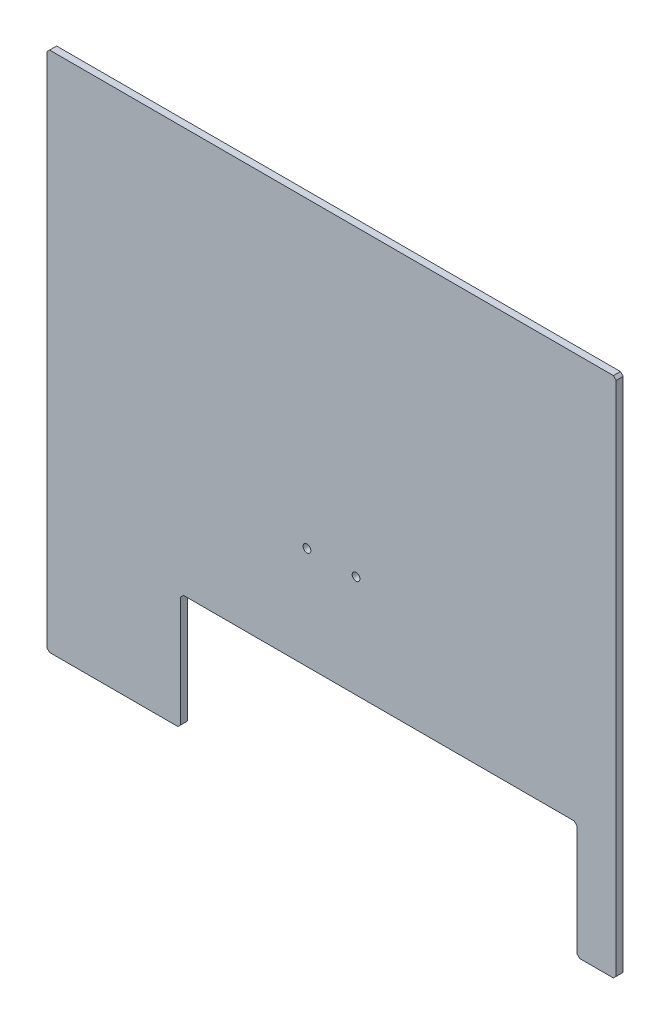
from build123d import *

# Parameters (mm, degrees)
SKETCH1_W            = 406
SKETCH1_H            = 372
BOSS_EXTRUDE1_DEPTH  = 5
SKETCH2_W            = 282.5
SKETCH2_H            = 83
CUT_EXTRUDE1_DEPTH   = 276.372475022
M5_CLEARANCE_HOLE1_D = 5.5
FILLET1_SIZE         = 2


with BuildPart() as part:
    # Sketch1 → Boss-Extrude1 (new body)
    with BuildSketch(Plane.XY):
        Rectangle(SKETCH1_W, SKETCH1_H)
    extrude(amount=BOSS_EXTRUDE1_DEPTH)

    # Sketch2 → Cut-Extrude1 (cut, through all)
    with BuildSketch(Plane.XY.offset(5)):
        with Locations((33.75, -144.5)):
            Rectangle(SKETCH2_W, SKETCH2_H)
    extrude(amount=-CUT_EXTRUDE1_DEPTH, mode=Mode.SUBTRACT)

    # M5 Clearance Hole1 (through all)
    with Locations(Plane.XY.offset(5)):
        with Locations((-17.5, -30), (17.5, -30)):
            Hole(M5_CLEARANCE_HOLE1_D / 2)

    # Fillet1
    fillet1_edges = [part.edges().sort_by_distance(p)[0] for p in [
        (-107.5, -186, 2.5),
        (-107.5, -103, 2.5),
        (175, -103, 2.5),
        (175, -186, 2.5),
        (-203, 186, 2.5),
        (203, 186, 2.5),
        (203, -186, 2.5),
        (-203, -186, 2.5),
    ]]
    chamfer(fillet1_edges, length=FILLET1_SIZE)


solid = part.part
